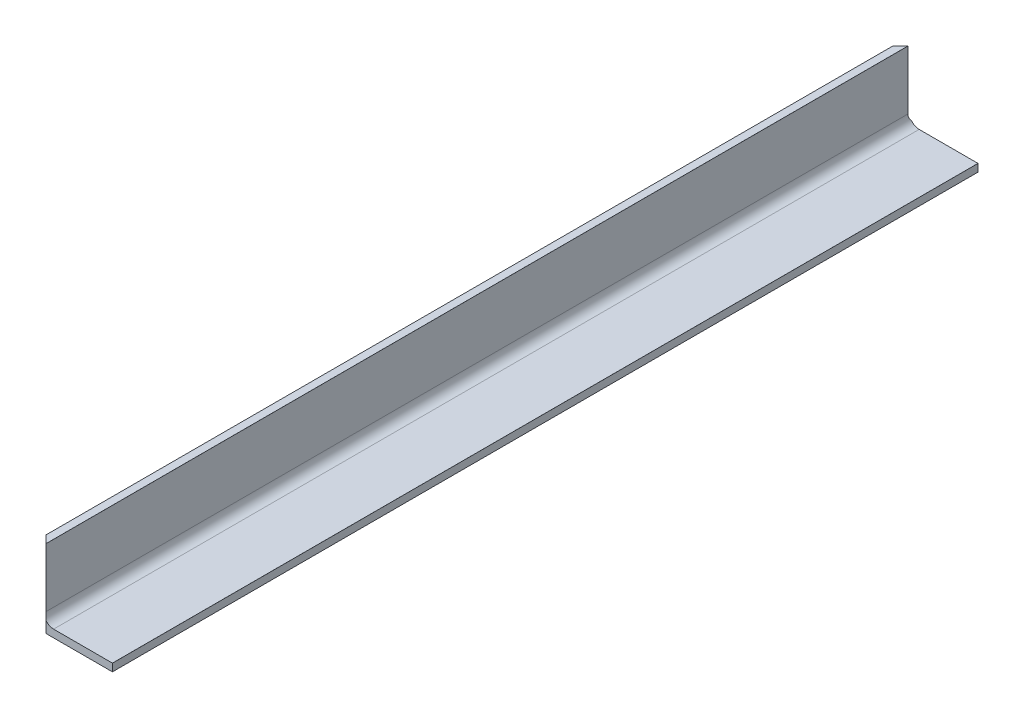
SolidWorks part; units mm, degrees
material "热轧等边角钢 Q235A"
ref_plane "前视基准面" through (0, 0, 0) normal (0, 0, 1) x (1, 0, 0)
ref_plane "上视基准面" through (0, 0, 0) normal (0, 1, 0) x (1, 0, 0)
ref_plane "右视基准面" through (0, 0, 0) normal (1, 0, 0) x (0, 0, -1)
sketch "草图1" plane through (0, 0, 0) normal (0, 0, 1) x (1, 0, 0)
  line L0 (0, 0) -> (0, 40)
  line L1 (0, 40) -> (3.99, 40)
  line L2 (4, 39.99) -> (4, 9)
  line L3 (9, 4) -> (39.99, 4)
  line L4 (40, 3.99) -> (40, 0)
  line L5 (40, 0) -> (0, 0)
  arc A0 (4, 39.99) -> (3.99, 40) centre (3.99, 39.99) ccw
  arc A1 (9, 4) -> (4, 9) centre (9, 9) cw
  arc A2 (40, 3.99) -> (39.99, 4) centre (39.99, 3.99) ccw
  point P9 (4, 40)
  point P14 (40, 4)
extrude "拉伸1" add sketch "草图1" along normal blind 456
sketch "草图2" plane through (0, 40, 0) normal (0, 1, 0) x (1, 0, 0)
  line L0 (5, -456) -> (0, -451)
  line L1 (3.99, -456) -> (0, -456) construction
  line L3 (0, -456) -> (0, 0) construction
  line L4 (0, -451) -> (0, -456)
  line L5 (0, -456) -> (5, -456)
  line L6 (0, 0) -> (0, -5)
  line L7 (0, -5) -> (5, 0)
  line L8 (39.99, 0) -> (9, 0) construction
  line L9 (5, 0) -> (0, 0)
  dimension "D1" = 5
  dimension "D2" = 5
  dimension "D3" = 5
  dimension "D4" = 5
  dimension "D5" = 0
extrude "切除-拉伸1" cut sketch "草图2" against normal blind 40
equation "\"D2@草图1\" = \"D1@草图1\""
equation "\"D4@草图1\" = \"D3@草图1\""
equation "\"D7@草图1\" = \"D5@草图1\""
